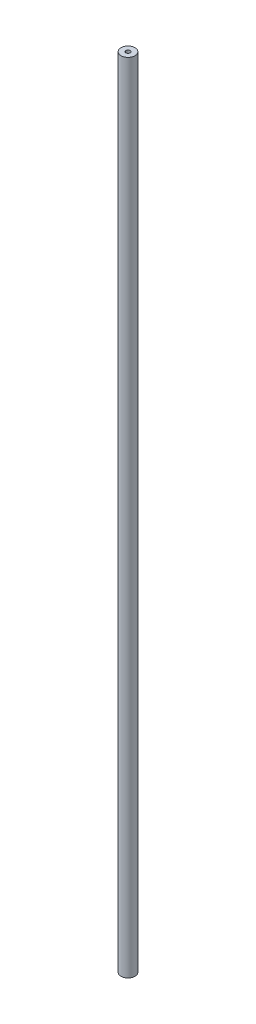
from build123d import *

# Parameters (mm, degrees)
SKETCH_1_R              = 20
EXTRUDE_1_DEPTH         = 2286
HOLE_WIZARD_M14_1_D     = 12
HOLE_WIZARD_M14_1_DEPTH = 34
HOLE_WIZARD_M14_1_TIP   = 3.605163714
HOLE_WIZARD_M14_2_D     = 12
HOLE_WIZARD_M14_2_DEPTH = 34
HOLE_WIZARD_M14_2_TIP   = 3.605163714


with BuildPart() as part:
    # 草图1 → 凸台-拉伸1 (new body)
    with BuildSketch(Plane(origin=(0, 0, 0), x_dir=(1, 0, 0), z_dir=(0, 1, 0))):
        with Locations(Location((0, 0, 0), (0, 0, 270))):
            Circle(SKETCH_1_R)
    extrude(amount=EXTRUDE_1_DEPTH)

    # M14 螺纹孔1
    with Locations(Plane(origin=(0, 2286, 0), x_dir=(1, 0, 0), z_dir=(0, 1, 0))):
        with Locations((0, 0)):
            Hole(HOLE_WIZARD_M14_1_D / 2, depth=HOLE_WIZARD_M14_1_DEPTH)
            with Locations((0, 0, -(HOLE_WIZARD_M14_1_DEPTH + HOLE_WIZARD_M14_1_TIP / 2))):  # 118° drill point
                Cone(0, HOLE_WIZARD_M14_1_D / 2, HOLE_WIZARD_M14_1_TIP, mode=Mode.SUBTRACT)

    # M14 螺纹孔2
    with Locations(Plane(origin=(0, 0, 0), x_dir=(-1, 0, 0), z_dir=(0, -1, 0))):
        with Locations((0, 0)):
            Hole(HOLE_WIZARD_M14_2_D / 2, depth=HOLE_WIZARD_M14_2_DEPTH)
            with Locations((0, 0, -(HOLE_WIZARD_M14_2_DEPTH + HOLE_WIZARD_M14_2_TIP / 2))):  # 118° drill point
                Cone(0, HOLE_WIZARD_M14_2_D / 2, HOLE_WIZARD_M14_2_TIP, mode=Mode.SUBTRACT)


solid = part.part
